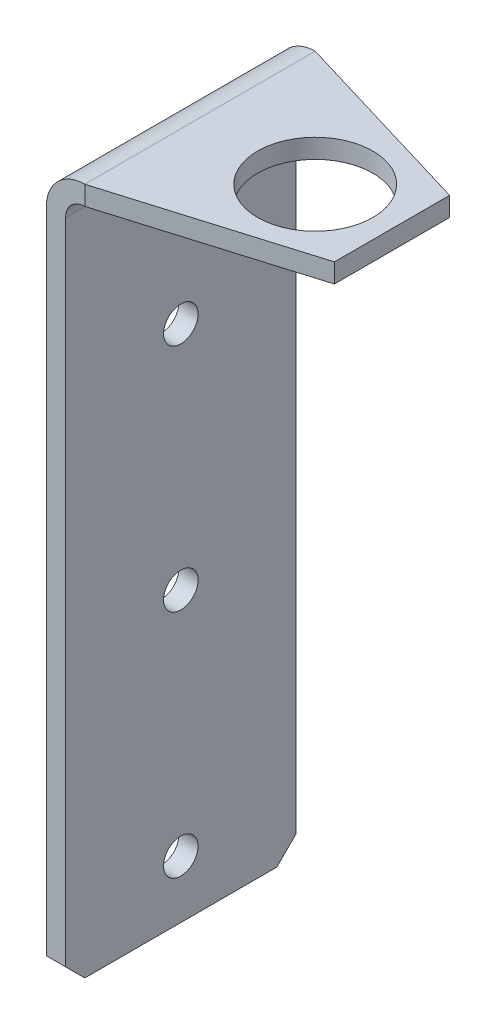
SolidWorks part; units mm, degrees
material "1023 碳钢板 (SS)"
ref_plane "Front Plane" through (0, 0, 0) normal (0, 0, 1) x (1, 0, 0)
ref_plane "Top Plane" through (0, 0, 0) normal (0, 1, 0) x (1, 0, 0)
ref_plane "Right Plane" through (0, 0, 0) normal (1, 0, 0) x (0, 0, -1)
sketch "Sketch1" plane through (0, 0, 0) normal (0, 0, 1) x (1, 0, 0)
  line L0 (0, 0) -> (0, 174)
  line L1 (10, 184) -> (60, 184)
  line L2 (5, 0) -> (5, 174)
  line L3 (10, 179) -> (60, 179)
  line L6 (0, 0) -> (5, 0)
  line L7 (60, 184) -> (60, 179)
  arc A0 (0, 174) -> (10, 184) centre (10, 174) cw
  arc A1 (5, 174) -> (10, 179) centre (10, 174) cw
  point P6 (0, 184)
  dimension "D3" = 10
  dimension "D1" = 60
  dimension "D2" = 184
  dimension "D4" = 5
extrude "Boss-Extrude1" add sketch "Sketch1" along normal blind 60
sketch "Sketch3" plane through (5, 0, 0) normal (1, 0, 0) x (0, 0, -1)
  line L0 (-60, 0) -> (0, 0) construction
  circle A0 centre (-30, 15) radius 4.5
  circle A1 centre (-30, 75) radius 4.5
  circle A2 centre (-30, 135) radius 4.5
  dimension "D1" = 9
  dimension "D2" = 15
  dimension "D3" = 3
chamfer "Chamfer1" distance 5 angle 45 2 edges at (2.5, 0, 0) (2.5, 0, 60)
sketch "Sketch5" plane through (0, 184, 0) normal (0, 1, 0) x (1, 0, 0)
  line L0 (60, -60) -> (60, 0) construction
  line L1 (0, -60) -> (0, 0) construction
  circle A0 centre (40, -30) radius 15
  point P5 (60, -30)
  dimension "D2" = 30
  dimension "D1" = 40
extrude "Cut-Extrude1" cut sketch "Sketch5" against normal blind 60
sketch "Sketch6" plane through (0, 184, 0) normal (0, 1, 0) x (1, 0, 0)
  line L0 (10, 0) -> (60, -15)
  line L1 (60, -60) -> (60, 0) construction
  line L3 (60, -45) -> (10, -60)
  line L5 (10, 0) -> (60, 0)
  line L6 (60, 0) -> (60, -15)
  line L7 (60, -45) -> (60, -60)
  line L8 (60, -60) -> (10, -60)
  dimension "D1" = 30
  dimension "D2" = 15
extrude "Cut-Extrude2" cut sketch "Sketch6" against normal blind 60
extrude "Cut-Extrude3" cut sketch "Sketch3" against normal blind 10
